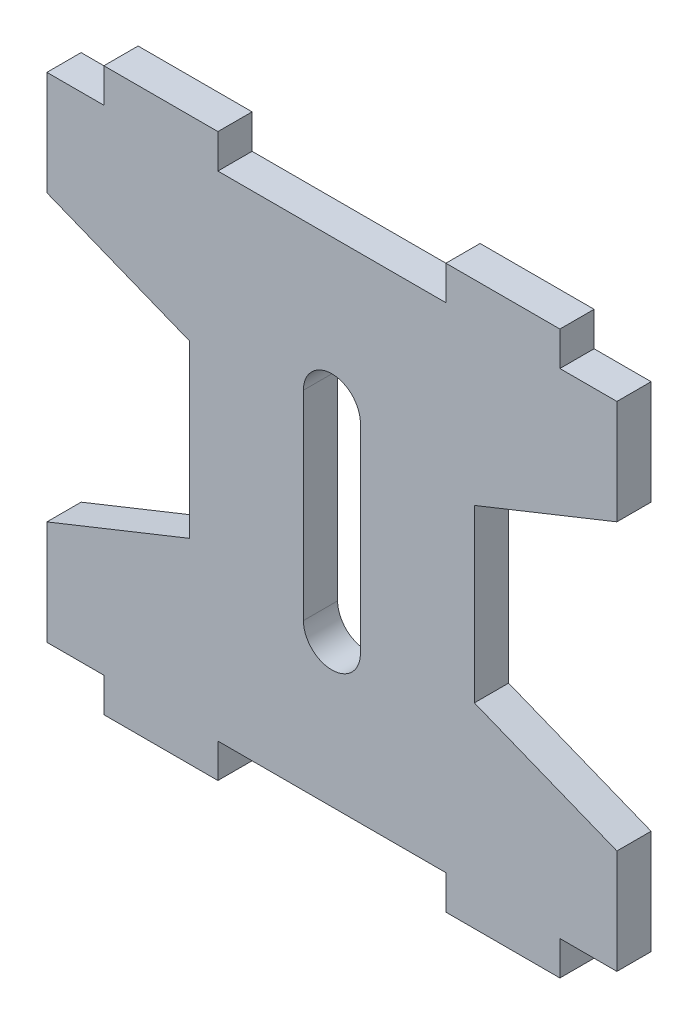
from build123d import *

# Parameters (mm, degrees)
EXTRUDE_1_DEPTH = 3


with BuildPart() as part:
    # 草图1 → 凸台-拉伸1 (new body)
    with BuildSketch(Plane.XY):
        Polygon((-25.609151467, -21.768855911), (-20.609151467, -21.768855911), (-20.609151467, -24.768855911), (-10.609151467, -24.768855911), (-10.609151467, -21.768855911), (9.390848533, -21.768855911), (9.390848533, -24.768855911), (19.390848533, -24.768855911), (19.390848533, -21.768855911), (24.390848533, -21.768855911), (24.390848533, -12.618855911), (11.890848533, -7.618855911), (11.890848533, 7.381144089), (24.390848533, 12.381144089), (24.390848533, 21.531144089), (19.390848533, 21.531144089), (19.390848533, 24.531144089), (9.390848533, 24.531144089), (9.390848533, 21.531144089), (-10.609151467, 21.531144089), (-10.609151467, 24.531144089), (-20.609151467, 24.531144089), (-20.609151467, 21.531144089), (-25.609151467, 21.531144089), (-25.609151467, 12.381144089), (-13.109151467, 7.381144089), (-13.109151467, -7.618855911), (-25.609151467, -12.618855911), align=None)
        with BuildLine():
            Line((1.890848533, 8.631144089), (1.890848533, -8.868855911))
            ThreePointArc((1.890848533, -8.868855911), (-0.609151467, -11.368855911), (-3.109151467, -8.868855911))
            Line((-3.109151467, -8.868855911), (-3.109151467, 8.631144089))
            ThreePointArc((-3.109151467, 8.631144089), (-0.609151467, 11.131144089), (1.890848533, 8.631144089))
        make_face(mode=Mode.SUBTRACT)
    extrude(amount=EXTRUDE_1_DEPTH)


solid = part.part
